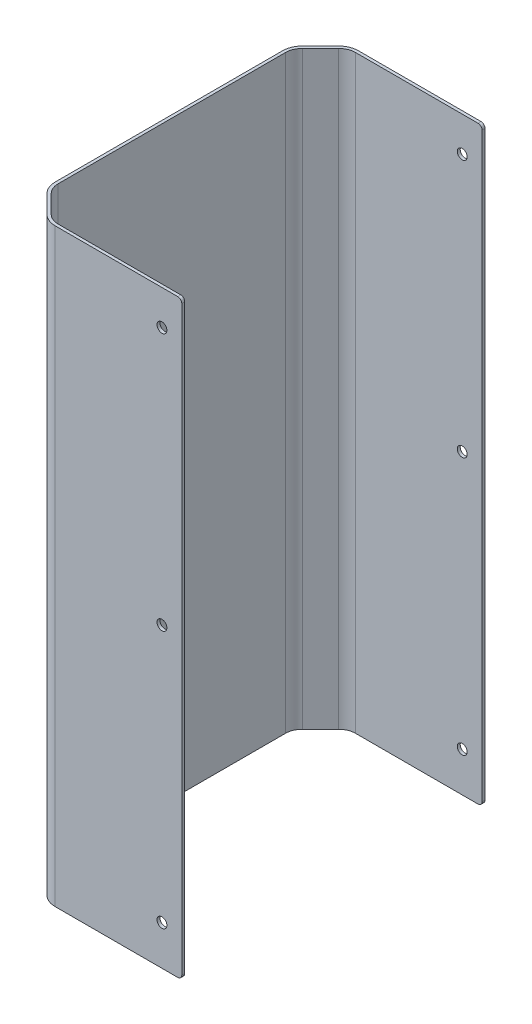
SolidWorks part; units mm, degrees
material "Q235"
ref_plane "前视基准面" through (0, 0, 0) normal (0, 0, 1) x (1, 0, 0)
ref_plane "上视基准面" through (0, 0, 0) normal (0, 1, 0) x (1, 0, 0)
ref_plane "右视基准面" through (0, 0, 0) normal (1, 0, 0) x (0, 0, -1)
sketch "草图1" plane through (0, 0, 0) normal (0, 0, 1) x (1, 0, 0)
  line L0 (0, 0) -> (-90, 0)
  line L1 (0, 0) -> (0, 490)
  line L2 (0, 490) -> (-70, 490)
  line L3 (5922.5, 0) -> (-90, 0) construction
  arc A0 (-70, 490) -> (-90, 0) centre (5922.5, 0) ccw
  dimension "D1" = 490
  dimension "D2" = 90
  dimension "D3" = 70
extrude "凸台-拉伸1" [suppressed] add sketch "草图1" along normal mid plane 173
shell "抽壳1" [suppressed] thickness 1.5
sketch "草图2" plane through (0, 0, 0) normal (0, 1, 0) x (1, 0, 0)
  line L1 (-41.5, 76.5) -> (41.5, 76.5)
  line L2 (-41.5, 76.5) -> (-41.5, -76.5)
  line L3 (-41.5, -76.5) -> (41.5, -76.5)
  line L4 (41.5, 76.5) -> (41.5, -76.5)
  line L5 (-41.5, 76.5) -> (41.5, -76.5) construction
  line L6 (-41.5, -76.5) -> (41.5, 76.5) construction
  point P0 (0, 0)
  dimension "D1" = 83
  dimension "D2" = 153
extrude "凸台-拉伸2" add sketch "草图2" against normal blind 297.5
chamfer "倒角1" distance 15 angle 45 2 edges at (-41.5, -148.75, -76.5) (-41.5, -148.75, 76.5)
fillet "圆角1" radius 10 4 edges at (-41.5, -148.75, -61.5) (-26.5, -148.75, -76.5) (-41.5, -148.75, 61.5) (-26.5, -148.75, 76.5)
shell "抽壳2" thickness 1.5
hole_wizard "Ø5.0 (5) 直径孔1" positions "草图4" profile "草图3" hole size "Ø5.0" standard "GB" end condition through all
sketch "草图4" plane through (0, 0, 76.5) normal (0, 0, 1) x (1, 0, 0)
  line L1 (31.5, -17.5) -> (31.5, -147.5) construction
  line L2 (31.5, -147.5) -> (31.5, -277.5) construction
  line L10 (41.5, -297.5) -> (41.5, 0) construction
  line L11 (-22.3579, -297.5) -> (41.5, -297.5) construction
  point P2 (31.5, -17.5)
  point P4 (31.5, -147.5)
  point P6 (31.5, -277.5)
  dimension "D1" = 10
  dimension "D2" = 130
  dimension "D3" = 20
sketch "草图3" plane through (31.5, -17.5, 76.5) normal (1, 0, 0) x (0, -1, 0)
  line L0 (0, 0) -> (0, 153)
  line L1 (0, 153) -> (2.5, 153)
  line L2 (2.5, 153) -> (2.5, 0)
  line L5 (2.5, 0) -> (0, 0)
  line L11 (0, -6.35) -> (0, 107.95) construction
  dimension "通孔孔直径" = 5
  dimension "通孔孔深度" = 153
fillet "圆角2" radius 2 4 edges at (41.5, -297.5, -75.75) (41.5, -297.5, 75.75) (41.5, 0, 75.75) (41.5, 0, -75.75)
sketch "草图5" plane through (0, 0, 76.5) normal (0, 0, -1) x (-1, 0, 0)
  line L0 (3.5, 46.3037) -> (3.5, -25) construction
  line L1 (16, 46.3037) -> (16, -25)
  line L2 (-9, 46.3037) -> (-9, -25)
  line L3 (-39.5, 0) -> (22.3579, 0) construction
  line L4 (-41.5, -295.5) -> (-41.5, -2) construction
  arc A0 (16, 46.3037) -> (-9, 46.3037) centre (3.5, 46.3037) ccw
  arc A1 (-9, -25) -> (16, -25) centre (3.5, -25) ccw
  point P2 (3.5, 10.6519)
  dimension "D1" = 25
  dimension "D2" = 25
  dimension "D3" = 45
extrude "切除-拉伸1" [suppressed] cut sketch "草图5" along normal blind 10
sketch "草图6" plane through (-41.5, 0, 0) normal (-1, 0, 0) x (0, 0, 1)
  line L0 (0, -282.5) -> (0, -312.5) construction
  line L1 (-57.3579, -297.5) -> (57.3579, -297.5) construction
  line L2 (10, -282.5) -> (10, -312.5)
  line L3 (-10, -282.5) -> (-10, -312.5)
  arc A0 (10, -282.5) -> (-10, -282.5) centre (0, -282.5) ccw
  arc A1 (-10, -312.5) -> (10, -312.5) centre (0, -312.5) ccw
  point P5 (0, -297.5)
  dimension "D2" = 15
  dimension "D1" = 20
extrude "切除-拉伸2" [suppressed] cut sketch "草图6" against normal blind 10
